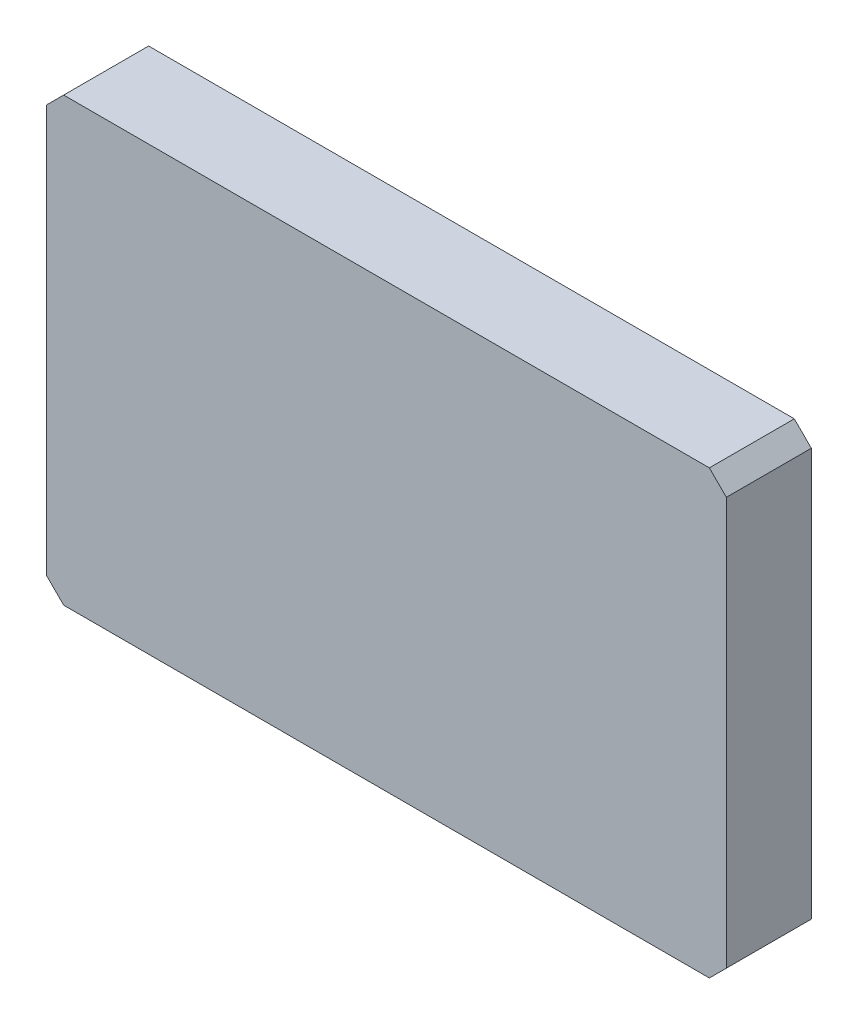
from build123d import *

# Parameters (mm, degrees)
SKETCH_1_W      = 200
SKETCH_1_H      = 130
EXTRUDE_1_DEPTH = 25
CHAMFER_1_SIZE  = 5


with BuildPart() as part:
    # 草图1 → 凸台-拉伸1 (new body)
    with BuildSketch(Plane.XY):
        Rectangle(SKETCH_1_W, SKETCH_1_H)
    extrude(amount=EXTRUDE_1_DEPTH)

    # 倒角1
    chamfer_1_edges = [part.edges().sort_by_distance(p)[0] for p in [
        (100, -65, 12.5),
        (-100, -65, 12.5),
        (-100, 65, 12.5),
        (100, 65, 12.5),
    ]]
    chamfer(chamfer_1_edges, length=CHAMFER_1_SIZE)


solid = part.part
